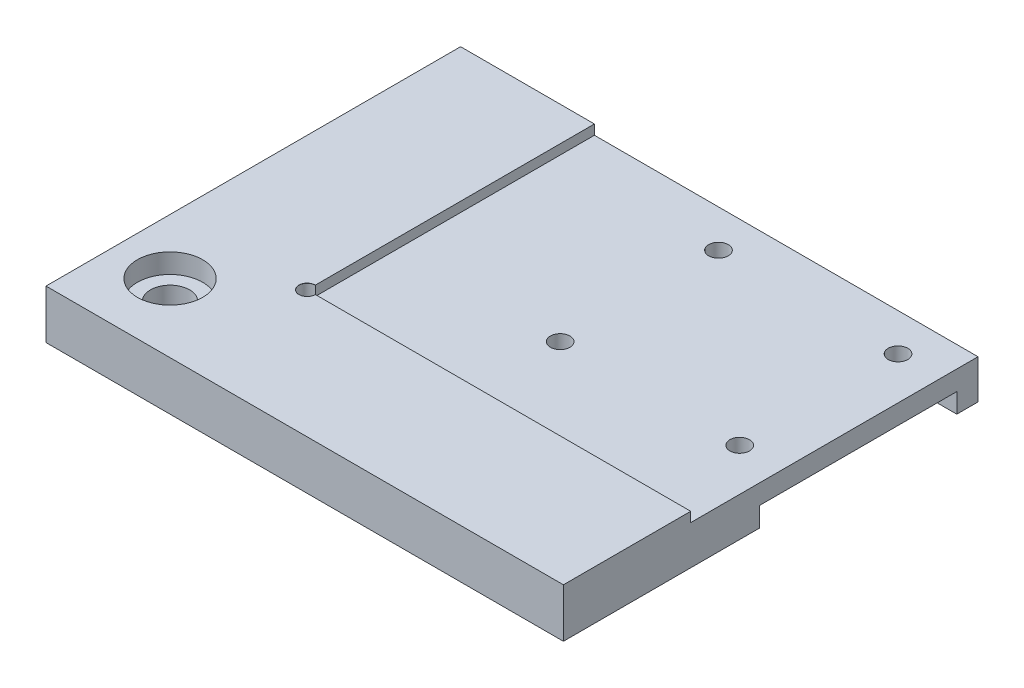
SolidWorks part; units mm, degrees
ref_plane "Front Plane" through (0, 0, 0) normal (0, 0, 1) x (1, 0, 0)
ref_plane "Top Plane" through (0, 0, 0) normal (0, 1, 0) x (1, 0, 0)
ref_plane "Right Plane" through (0, 0, 0) normal (1, 0, 0) x (0, 0, -1)
other "Configuration Table"
sketch "Sketch1" plane through (0, 0, 0) normal (0, 1, 0) x (1, 0, 0)
  line L1 (-79.25, 63.5) -> (79.25, 63.5)
  line L2 (-79.25, 63.5) -> (-79.25, -63.5)
  line L3 (-79.25, -63.5) -> (79.25, -63.5)
  line L4 (79.25, 63.5) -> (79.25, -63.5)
  line L5 (-79.25, 63.5) -> (79.25, -63.5) construction
  line L6 (-79.25, -63.5) -> (79.25, 63.5) construction
  point P0 (0, 0)
  dimension "D1" = 158.5
  dimension "D2" = 127
extrude "Boss-Extrude1" add sketch "Sketch1" along normal blind 15
sketch "Sketch2" plane through (0, 15, 0) normal (0, 1, 0) x (1, 0, 0)
  line L1 (79.25, 63.5) -> (-38.25, 63.5)
  line L2 (79.25, 63.5) -> (79.25, -24.5)
  line L3 (79.25, -24.5) -> (-38.25, -24.5)
  line L4 (-38.25, 63.5) -> (-38.25, -24.5)
  dimension "D1" = 88
  dimension "D2" = 117.5
extrude "Cut-Extrude1" cut sketch "Sketch2" against normal blind 3
sketch "Sketch3" plane through (0, 0, 0) normal (0, -1, 0) x (1, 0, 0)
  line L0 (79.25, 63.5) -> (79.25, -63.5) construction
  line L1 (79.25, -57) -> (-1.75, -57)
  line L2 (79.25, -57) -> (79.25, 3.5)
  line L3 (79.25, 3.5) -> (-1.75, 3.5)
  line L4 (-1.75, -57) -> (-1.75, 3.5)
  line L5 (79.25, -63.5) -> (-79.25, -63.5) construction
  dimension "D1" = 6.5
  dimension "D2" = 67
  dimension "D3" = 81
extrude "Cut-Extrude2" cut sketch "Sketch3" against normal blind 6
sketch "Sketch4" plane through (0, 0, 0) normal (0, 0, 1) x (1, 0, 0)
  line L0 (-1.75, 6) -> (79.25, 6) construction
  line L1 (-1.75, 0) -> (5.25, 0)
  line L2 (-1.75, 0) -> (-1.75, 6)
  line L3 (-1.75, 6) -> (5.25, 6)
  line L4 (5.25, 0) -> (5.25, 6)
  dimension "D1" = 7
extrude "Cut-Extrude3" cut sketch "Sketch4" against normal through all
sketch "Sketch5" plane through (0, 15, 0) normal (0, 1, 0) x (1, 0, 0)
  line L0 (79.25, 63.5) -> (-38.25, 63.5) construction
  line L1 (11.25, 52) -> (66.25, 52) construction
  line L2 (11.25, 52) -> (11.25, 3.5) construction
  line L3 (11.25, 3.5) -> (66.25, 3.5) construction
  line L4 (66.25, 52) -> (66.25, 3.5) construction
  line L5 (11.25, 52) -> (66.25, 3.5) construction
  line L6 (11.25, 3.5) -> (66.25, 52) construction
  line L7 (79.25, -24.5) -> (79.25, 63.5) construction
  circle A0 centre (11.25, 52) radius 3
  circle A1 centre (66.25, 52) radius 3
  circle A2 centre (66.25, 3.5) radius 3
  circle A3 centre (11.25, 3.5) radius 3
  point P0 (38.75, 27.75)
  dimension "D5" = 6
  dimension "D1" = 11.5
  dimension "D2" = 48.5
  dimension "D3" = 13
  dimension "D4" = 55
extrude "Cut-Extrude4" cut sketch "Sketch5" against normal through all
sketch "Sketch6" plane through (0, 15, 0) normal (0, 1, 0) x (1, 0, 0)
  circle A0 centre (-62.25, -42.5) radius 10
  circle A1 centre (11.25, 3.5) radius 3 construction
  dimension "D1" = 46
  dimension "D3" = 20
  dimension "D2" = 73.5
extrude "Cut-Extrude5" cut sketch "Sketch6" against normal blind 6
sketch "Sketch7" plane through (0, 9, 0) normal (0, 1, 0) x (1, 0, 0)
  circle A0 centre (-62.25, -42.5) radius 6
  dimension "D1" = 12
extrude "Cut-Extrude6" cut sketch "Sketch7" against normal through all
hole_wizard "Ø5.0mm blind dowel hole 1" positions "Sketch8" profile "Sketch9" hole size "Ø5.0" standard "GB"
sketch "Sketch8" plane through (0, 15, 0) normal (0, 1, 0) x (1, 0, 0)
  point P0 (-38.25, -24.5)
sketch "Sketch9" plane through (-38.25, 15, 24.5) normal (1, 0, 0) x (0, 0, 1)
  line L0 (0, 0) -> (0, 5.5022)
  line L1 (0, 5.5022) -> (2.5, 4)
  line L2 (2.5, 4) -> (2.5, 0.025)
  line L3 (2.5, 0.025) -> (2.525, 0)
  line L5 (2.525, 0) -> (0, 0)
  line L6 (-2.5, 0.025) -> (-2.525, 0) construction
  line L10 (0, 5.5022) -> (-2.5, 4) construction
  line L11 (0, -6.35) -> (0, 107.95) construction
  dimension "孔直径" = 5
  dimension "孔深度" = 4
  dimension "近端锥形沉头孔直径" = 5.05
  dimension "近端锥形沉头孔角度" = 90
  dimension "导头角度" = 118
